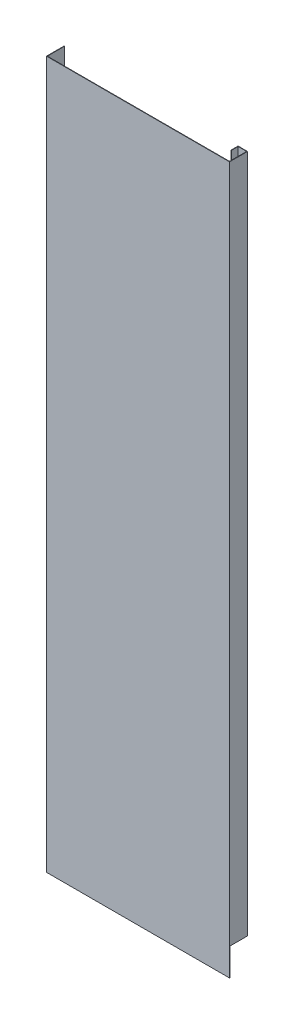
from build123d import *

# Parameters (mm, degrees)
EXTRUDE_THIN1_DEPTH = 1649
SKETCH5_W           = 22
SKETCH5_H           = 64
CUT_EXTRUDE2_DEPTH  = 41


with BuildPart() as part:
    # Sketch3 → Extrude-Thin1 (new body)
    with BuildSketch(Plane(origin=(0, 0, 0), x_dir=(1, 0, 0), z_dir=(0, 1, 0))):
        Polygon((0, 40), (0, 0), (425, 0), (425, 40), (405, 40), (405, 25), (404, 25), (404, 41), (426, 41), (426, -1), (-1, -1), (-1, 40), align=None)
    extrude(amount=EXTRUDE_THIN1_DEPTH)

    # Sketch5 → Cut-Extrude2 (cut)
    with BuildSketch(Plane(origin=(0, 0, -41), x_dir=(-1, 0, 0), z_dir=(0, 0, -1))):
        with Locations((-415, 32)):
            Rectangle(SKETCH5_W, SKETCH5_H)
    extrude(amount=-CUT_EXTRUDE2_DEPTH, mode=Mode.SUBTRACT)


solid = part.part
